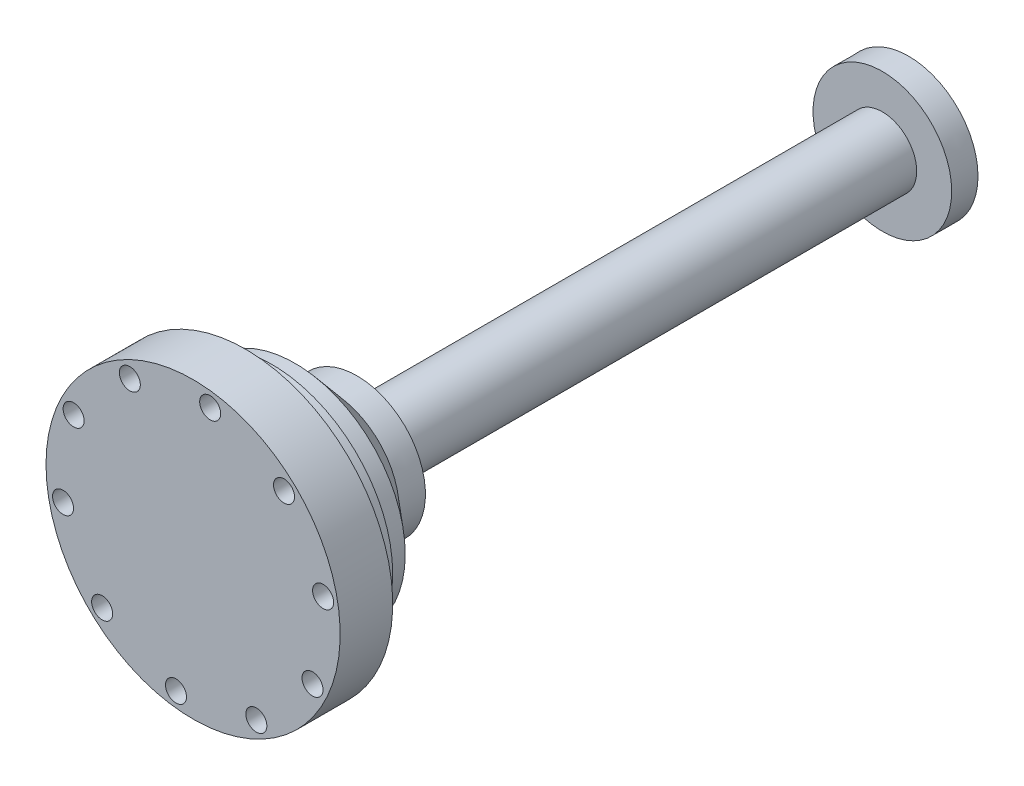
SolidWorks part; units mm, degrees
ref_plane "Front Plane" through (0, 0, 0) normal (0, 0, 1) x (1, 0, 0)
ref_plane "Top Plane" through (0, 0, 0) normal (0, 1, 0) x (1, 0, 0)
ref_plane "Right Plane" through (0, 0, 0) normal (1, 0, 0) x (0, 0, -1)
sketch "Sketch2" plane through (0, 0, 0) normal (0, 0, 1) x (1, 0, 0)
  line L0 (20, 68.8305) -> (20, 42.8305) construction
  line L1 (20, 70.8305) -> (20, 40.8305) construction
  circle A0 centre (20, 55.8305) radius 13 construction
ref_plane "Plane4" through (20, 0, 0) normal (-1, 0, 0) x (0, -1, 0)
sketch "Sketch4" plane through (20, 0, 0) normal (-1, 0, 0) x (0, -1, 0)
  line L0 (-76.8305, 0) -> (-76.8305, -4.3834)
  line L1 (-76.8305, -4.3834) -> (-68.8305, -11.2146)
  line L2 (-68.8305, -11.2146) -> (-69.0345, -121.2146)
  line L3 (-69.0345, -121.2146) -> (-55.8305, -121.2146)
  line L8 (-76.8305, 0) -> (-78.8305, 0)
  line L9 (-78.8305, 0) -> (-78.8305, -4.3834) construction
  line L10 (-78.8305, 0) -> (-78.8027, 15)
  line L11 (-78.8027, 15) -> (-55.8305, 15)
  line L12 (-55.8305, 15) -> (-55.8305, -121.2146)
  line L13 (-68.8305, 0) -> (-42.8305, 0) construction
  point P15 (-55.8305, 0)
  dimension "D1" = 15
revolve "Revolve1" add sketch "Sketch4" angle 360 about L12
sketch "Sketch5" plane through (20, 0, 0) normal (-1, 0, 0) x (0, -1, 0)
  line L0 (-42.6265, -121.2146) -> (-42.8305, -11.2146) construction
  line L1 (-36.1555, -116.2146) -> (-49.3015, -116.2146)
  line L2 (-36.1555, -116.2146) -> (-36.1555, -16.2146)
  line L3 (-36.1555, -16.2146) -> (-49.3015, -16.2146)
  line L4 (-49.3015, -116.2146) -> (-49.3015, -16.2146)
  line L5 (-36.1555, -116.2146) -> (-49.3015, -16.2146) construction
  line L6 (-36.1555, -16.2146) -> (-49.3015, -116.2146) construction
  line L7 (-69.0345, -121.2146) -> (-42.6265, -121.2146) construction
  line L8 (-55.8305, -11.2146) -> (-55.8305, -121.2146) construction
  line L9 (-68.8305, -11.2146) -> (-42.8305, -11.2146) construction
  point P0 (-42.7285, -66.2146)
  dimension "D1" = 5
revolve "Cut-Revolve1" cut sketch "Sketch5" angle 360 about L8
sketch "Sketch6" plane through (0, 0, 15) normal (0, 0, -1) x (-1, 0, 0)
  circle A1 centre (-20, 55.8305) radius 28
  circle A6 centre (-20, 55.8305) radius 28
  dimension "D1" = 0
extrude "Boss-Extrude1" add sketch "Sketch6" along normal blind 10
sketch "Sketch7" plane through (0, 0, 5) normal (0, 0, -1) x (-1, 0, 0)
  circle A0 centre (4.753, 51.2099) radius 2 construction
  circle A1 centre (4.753, 51.2099) radius 2
extrude "Cut-Extrude1" cut sketch "Sketch7" against normal blind 10
pattern_circular "CirPattern1" count 10 over 360 about axis through (20, 55.8305, 0) along (0, 0, 1) of "Cut-Extrude1"
